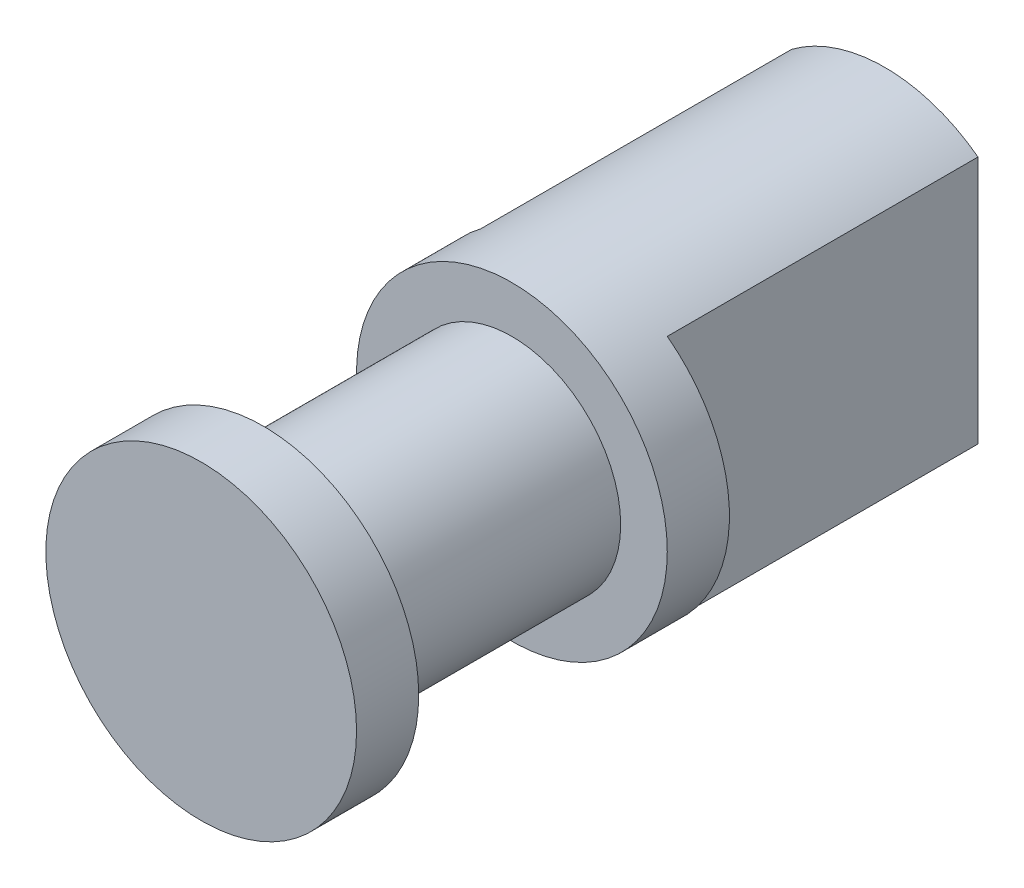
SolidWorks part; units mm, degrees
ref_plane "Front Plane" through (0, 0, 0) normal (0, 0, 1) x (1, 0, 0)
ref_plane "Top Plane" through (0, 0, 0) normal (0, 1, 0) x (1, 0, 0)
ref_plane "Right Plane" through (0, 0, 0) normal (1, 0, 0) x (0, 0, -1)
other "Configuration Table"
sketch "Sketch1" plane through (0, 0, 0) normal (0, 0, 1) x (1, 0, 0)
  circle A0 centre (0, 0) radius 2.5
  dimension "D1" = 5
extrude "Boss-Extrude1" add sketch "Sketch1" along normal blind 11
sketch "Sketch2" plane through (0, 0, 0) normal (0, 0, -1) x (-1, 0, 0)
  line L0 (-1.5, 2) -> (-1.5, -2)
  line L1 (1.5, 2) -> (1.5, -2)
  arc A0 (-1.5, -2) -> (1.5, -2) centre (0, 0) ccw
  arc A1 (1.5, 2) -> (-1.5, 2) centre (0, 0) ccw
  dimension "D3" = 2.5
  dimension "D1" = 1.5
  dimension "D2" = 1.5
extrude "Cut-Extrude1" cut sketch "Sketch2" against normal blind 5 flip side to cut
sketch "Sketch3" plane through (0, 0, 11) normal (0, 0, 1) x (1, 0, 0)
  circle A0 centre (0, 0) radius 2.5
  circle A1 centre (0, 0) radius 1.75
  dimension "D1" = 3.5
extrude "Cut-Extrude2" cut sketch "Sketch3" against normal blind 4 from offset 1
